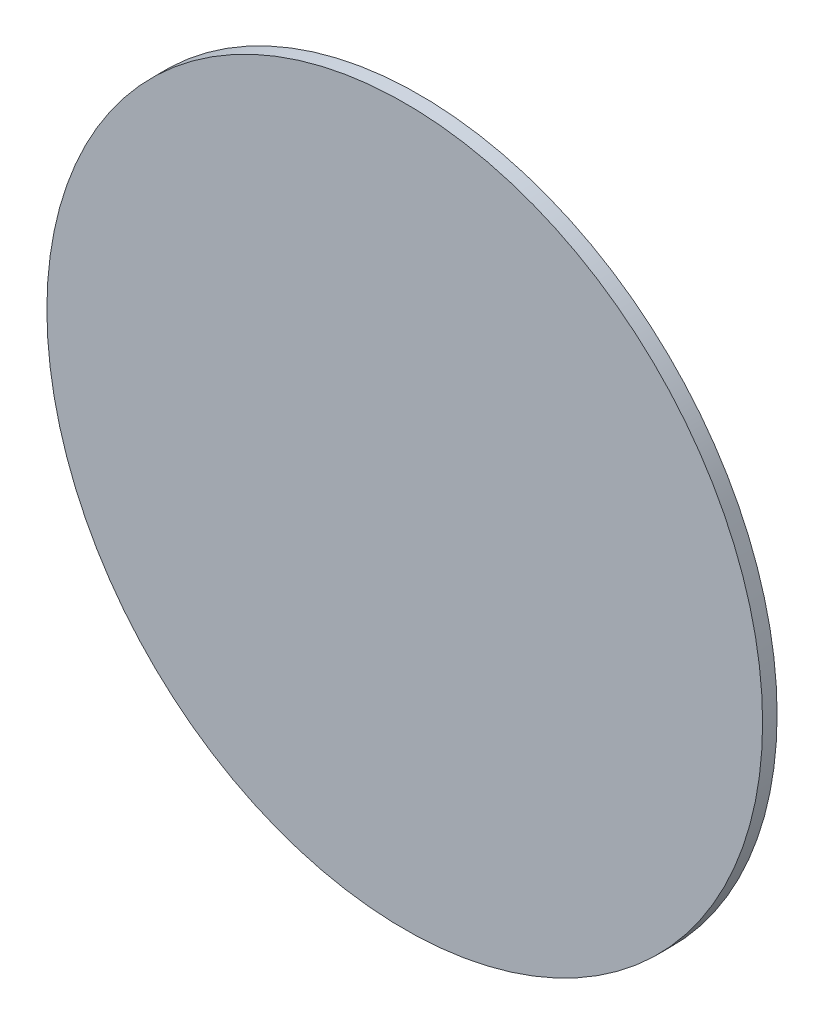
from build123d import *

# Parameters (mm, degrees)
SKETCH_1_R           = 74
BOSS_EXTRUDE_1_DEPTH = 3


with BuildPart() as part:
    # Sketch 1 → Boss-Extrude 1 (new body)
    with BuildSketch(Plane.XY):
        Circle(SKETCH_1_R)
    extrude(amount=BOSS_EXTRUDE_1_DEPTH)


solid = part.part
